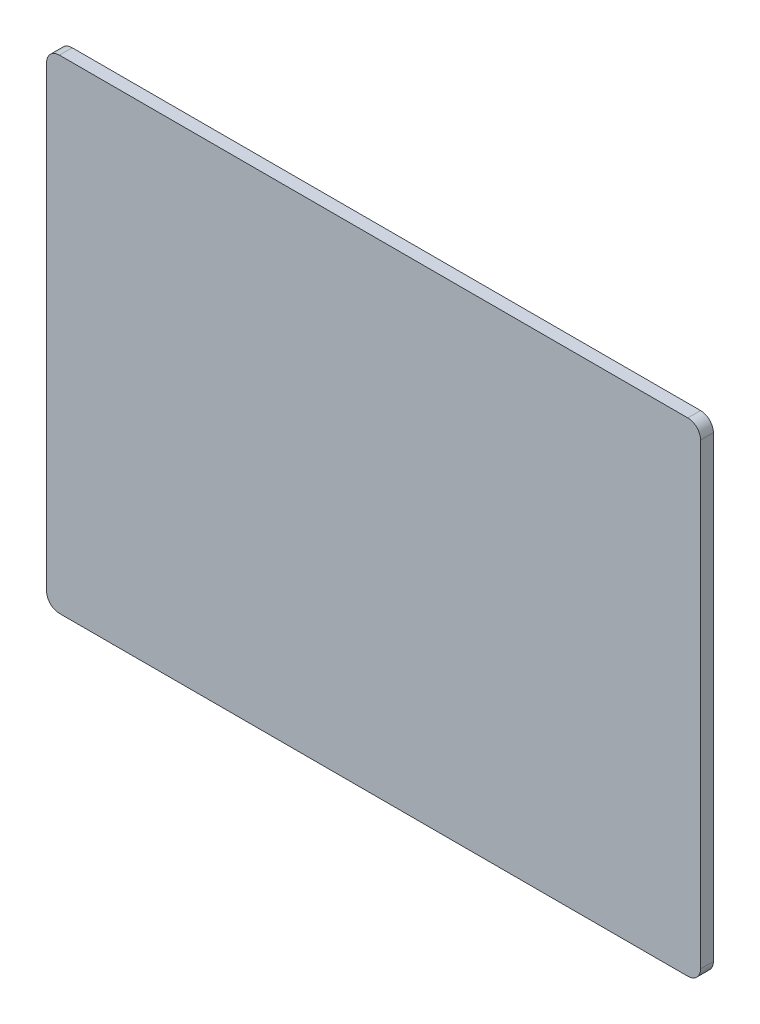
SolidWorks part; units mm, degrees
ref_plane "前视基准面" through (0, 0, 0) normal (0, 0, 1) x (1, 0, 0)
ref_plane "上视基准面" through (0, 0, 0) normal (0, 1, 0) x (1, 0, 0)
ref_plane "右视基准面" through (0, 0, 0) normal (1, 0, 0) x (0, 0, -1)
sketch "草图1" plane through (0, 0, 0) normal (0, 0, 1) x (1, 0, 0)
  line L1 (32.6337, 50.4476) -> (186.1337, 50.4476)
  line L2 (32.6337, 50.4476) -> (32.6337, -63.0524)
  line L3 (32.6337, -63.0524) -> (186.1337, -63.0524)
  line L4 (186.1337, 50.4476) -> (186.1337, -63.0524)
  dimension "D1" = 113.5
  dimension "D2" = 153.5
extrude "凸台-拉伸1" add sketch "草图1" along normal blind 3
fillet "圆角1" radius 3 4 edges at (32.6337, -63.0524, 1.5) (186.1337, -63.0524, 1.5) (186.1337, 50.4476, 1.5) (32.6337, 50.4476, 1.5)
